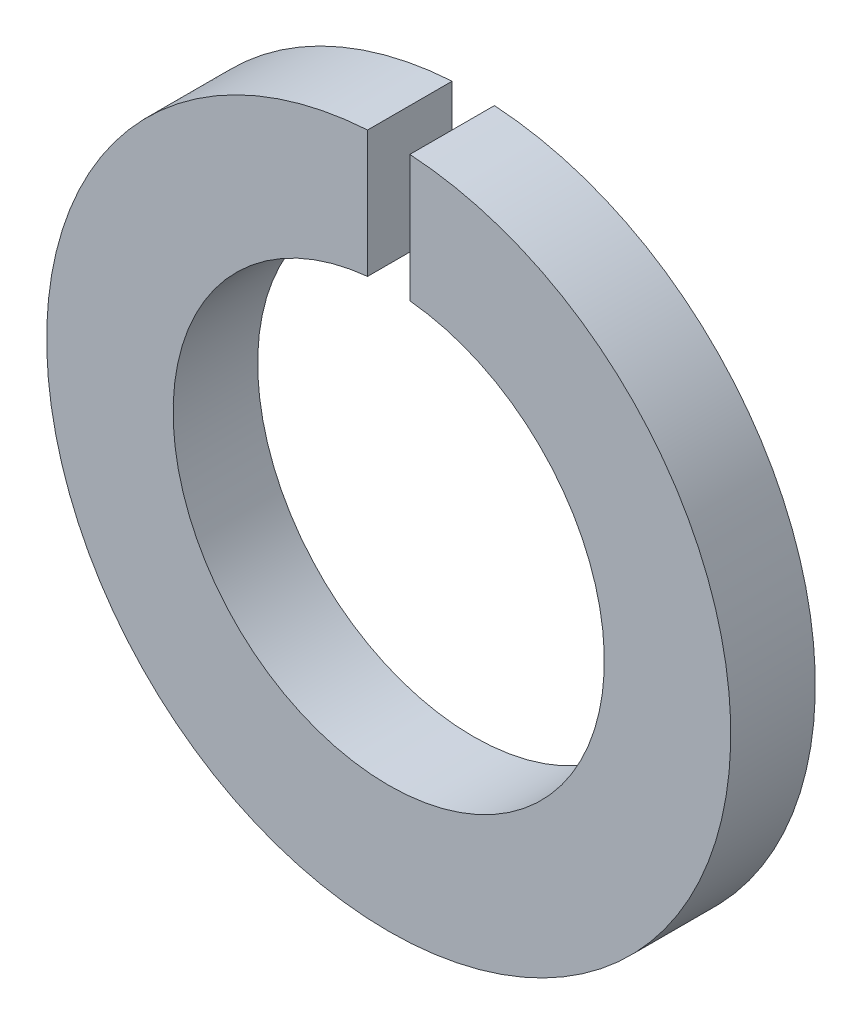
SolidWorks part; units mm, degrees
ref_plane "前视基准面" through (0, 0, 0) normal (0, 0, 1) x (1, 0, 0)
ref_plane "上视基准面" through (0, 0, 0) normal (0, 1, 0) x (1, 0, 0)
ref_plane "右视基准面" through (0, 0, 0) normal (1, 0, 0) x (0, 0, -1)
sketch "尺寸草图" plane through (0, 0, 0) normal (0, 0, 1) x (1, 0, 0)
  line L0 (0, 0) -> (0, 14.803) construction
  line L1 (-0.5, 8.0754) -> (-0.5, 5.0754)
  line L2 (0.5, 8.0754) -> (0.5, 5.0754)
  line L3 (0, 0) -> (2, 0) construction
  arc A0 (-0.5, 8.0754) -> (0.5, 8.0754) centre (0, 0) ccw
  arc A2 (-0.5, 5.0754) -> (0.5, 5.0754) centre (0, 0) ccw
  dimension "d" = 10.2
  dimension "m" = 1
  dimension "D4" = 0.5
  dimension "b" = 3
  dimension "s" = 2
extrude "拉伸1" add sketch "尺寸草图" along normal blind 2
